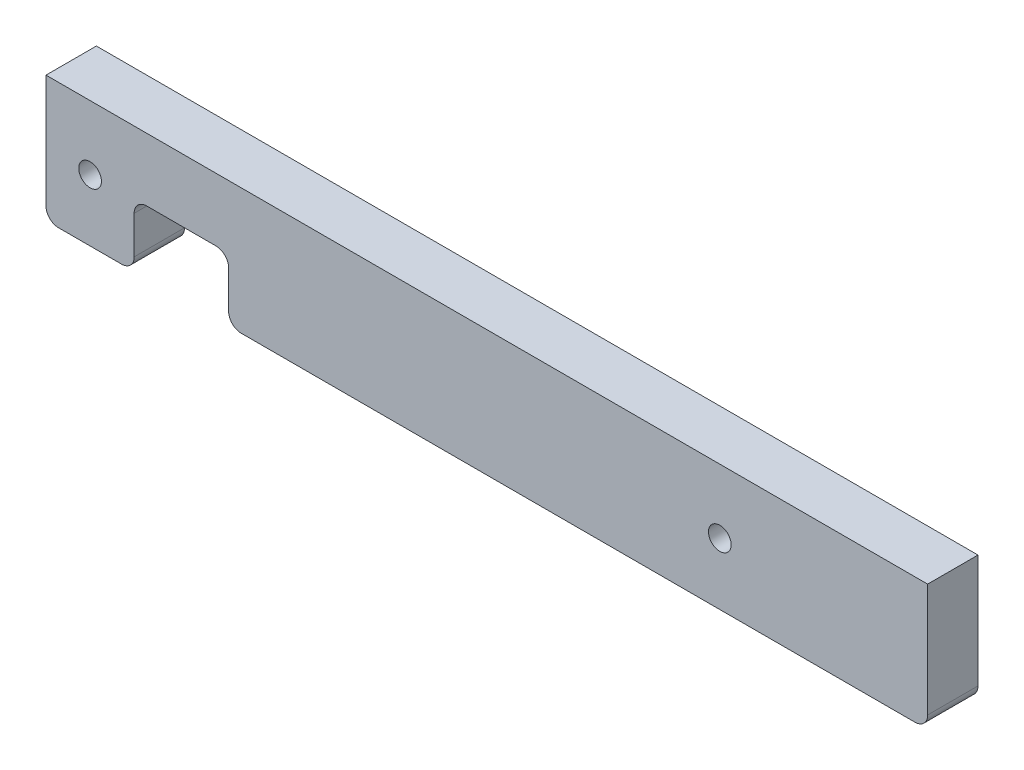
from build123d import *

# Parameters (mm, degrees)
SKETCH1_R           = 9
BOSS_EXTRUDE1_DEPTH = 40
FILLET1_R           = 10


with BuildPart() as part:
    # Sketch1 → Boss-Extrude1 (new body)
    with BuildSketch(Plane.XY):
        Polygon((70, 0), (70, 50), (145, 50), (145, 0), (700, 0), (700, 100), (0, 100), (0, 0), align=None)
        with Locations((35, 49)):
            Circle(SKETCH1_R, mode=Mode.SUBTRACT)
        with Locations((535, 49)):
            Circle(SKETCH1_R, mode=Mode.SUBTRACT)
    extrude(amount=BOSS_EXTRUDE1_DEPTH)

    # Fillet1
    fillet1_edges = [part.edges().sort_by_distance(p)[0] for p in [
        (145, 0, 20),
        (145, 50, 20),
        (70, 50, 20),
        (70, 0, 20),
        (0, 0, 20),
        (700, 0, 20),
    ]]
    fillet(fillet1_edges, radius=FILLET1_R)


solid = part.part
